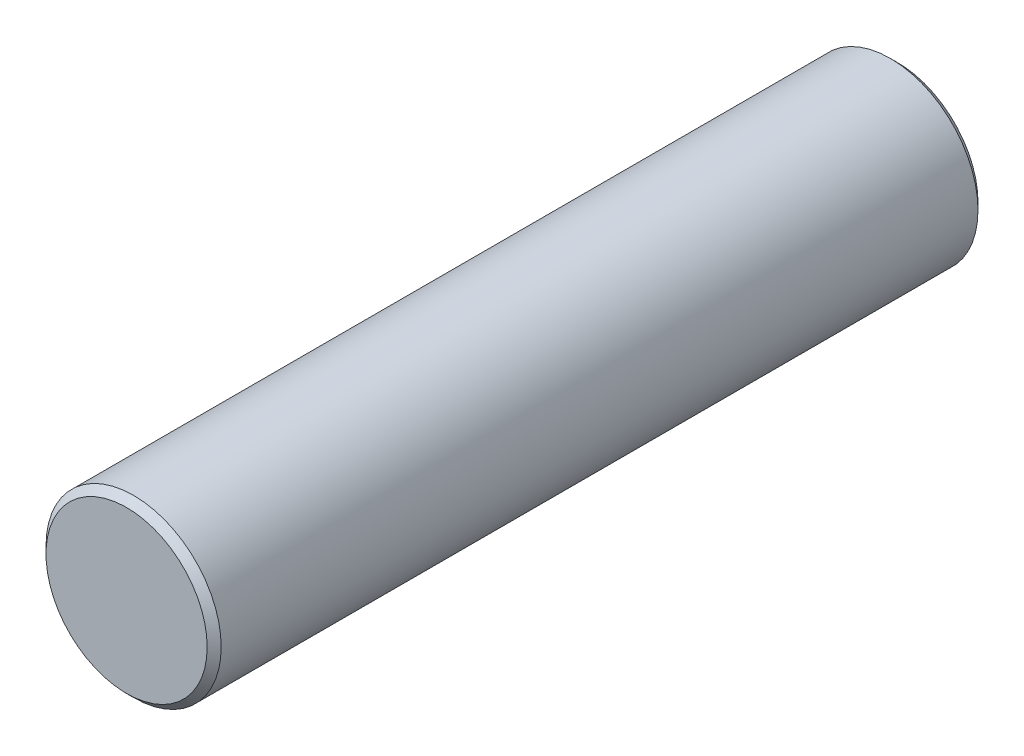
SolidWorks part; units mm, degrees
material "45"
ref_plane "Front Plane" through (0, 0, 0) normal (0, 0, 1) x (1, 0, 0)
ref_plane "Top Plane" through (0, 0, 0) normal (0, 1, 0) x (1, 0, 0)
ref_plane "Right Plane" through (0, 0, 0) normal (1, 0, 0) x (0, 0, -1)
sketch "Sketch1" plane through (0, 0, 0) normal (0, 0, 1) x (1, 0, 0)
  circle A0 centre (0, 0) radius 25
  dimension "D1" = 50
extrude "Boss-Extrude1" add sketch "Sketch1" along normal blind 220
chamfer "Chamfer1" distance 2 angle 45 2 edges at (25, 0, 0) (25, 0, 220)
